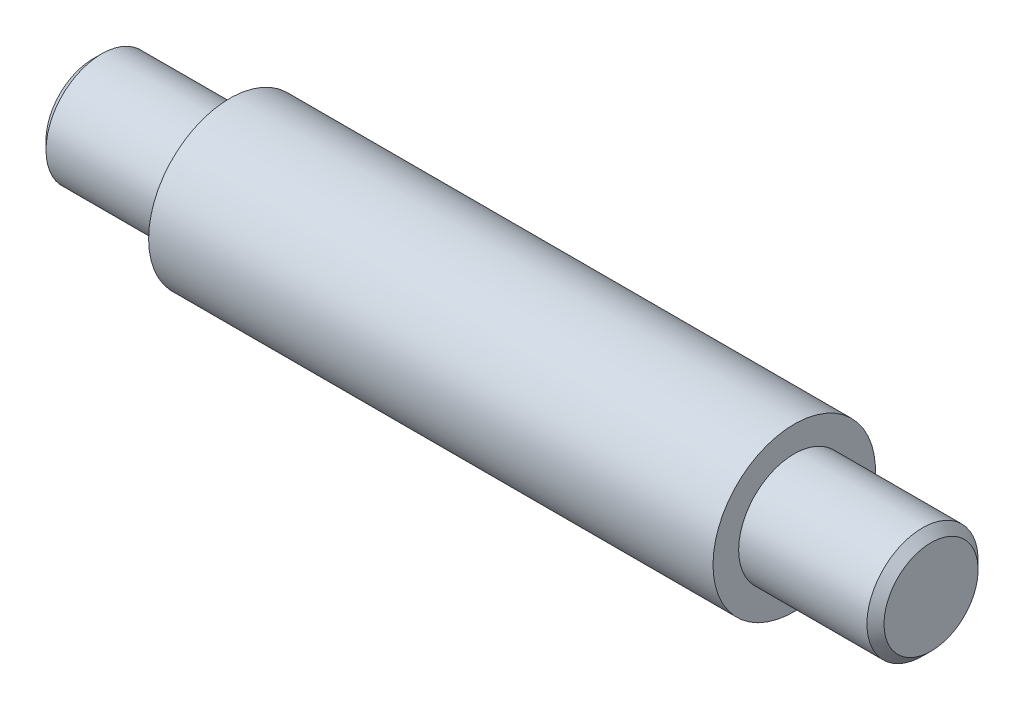
SolidWorks part; units mm, degrees
ref_plane "Front Plane" through (0, 0, 0) normal (0, 0, 1) x (1, 0, 0)
ref_plane "Top Plane" through (0, 0, 0) normal (0, 1, 0) x (1, 0, 0)
ref_plane "Right Plane" through (0, 0, 0) normal (1, 0, 0) x (0, 0, -1)
sketch "Sketch1" plane through (0, 0, 0) normal (0, 0, 1) x (1, 0, 0)
  line L0 (-1244.6, 0) -> (1244.6, 0)
  line L1 (1244.6, 0) -> (1244.6, 165.1)
  line L2 (1244.6, 165.1) -> (838.2, 165.1)
  line L3 (838.2, 165.1) -> (838.2, 241.3)
  line L4 (838.2, 241.3) -> (-838.2, 241.3)
  line L5 (-838.2, 241.3) -> (-838.2, 165.1)
  line L6 (-1244.6, 0) -> (-1244.6, 165.1)
  line L7 (-1244.6, 165.1) -> (-838.2, 165.1)
  dimension "D1" = 2489.2
  dimension "D2" = 165.1
  dimension "D3" = 1676.4
  dimension "D4" = 241.3
revolve "Revolve1" add sketch "Sketch1" angle 360 about L0
chamfer "Chamfer1" distance 25.4 angle 45 2 edges at (-1244.6, 0, 165.1) (1244.6, 0, 165.1)
